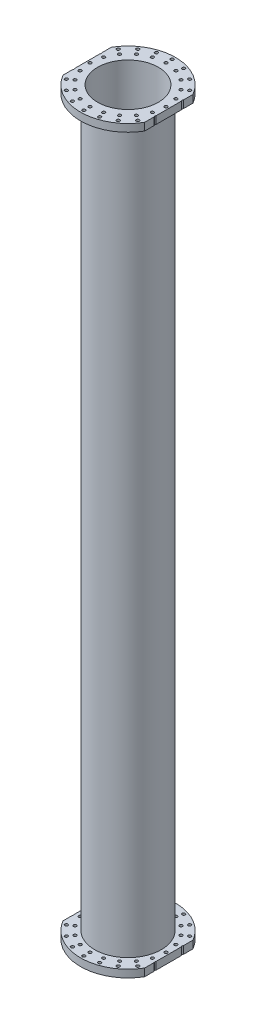
SolidWorks part; units mm, degrees
material "Q235B"
ref_plane "Front Plane" through (0, 0, 0) normal (0, 0, 1) x (1, 0, 0)
ref_plane "Top Plane" through (0, 0, 0) normal (0, 1, 0) x (1, 0, 0)
ref_plane "Right Plane" through (0, 0, 0) normal (1, 0, 0) x (0, 0, -1)
sketch "Sketch1" plane through (0, 0, 0) normal (0, 1, 0) x (1, 0, 0)
  line L1 (215, -400) -> (-215, -400)
  line L2 (215, -400) -> (215, 400)
  line L3 (215, 400) -> (-215, 400)
  line L4 (-215, -400) -> (-215, 400)
  line L5 (215, -400) -> (-215, 400) construction
  line L6 (215, 400) -> (-215, -400) construction
  circle A0 centre (0, 0) radius 250
  circle A1 centre (0, 0) radius 160
  dimension "D1" = 500
  dimension "D4" = 320
  dimension "D2" = 800
  dimension "D3" = 430
extrude "Boss-Extrude1" add sketch "Sketch1" along normal blind 40 contours L2 A0 L4 A1
sketch "Sketch2" plane through (0, 40, 0) normal (0, 1, 0) x (1, 0, 0)
  circle A0 centre (0, 0) radius 175.5
  circle A1 centre (0, 0) radius 160 construction
  circle A2 centre (0, 0) radius 160
  dimension "D1" = 351
extrude "Boss-Extrude2" add sketch "Sketch2" along normal blind 3817
hole_wizard "Ø16.0 (16) Diameter Hole1" positions "Sketch3" profile "Sketch4" hole size "Ø16.0" standard "GB" end condition up to next
sketch "Sketch3" plane through (0, 40, 0) normal (0, 1, 0) x (1, 0, 0)
  circle A0 centre (0, 0) radius 200 construction
  point P0 (200, 0)
  point P14 (190.2113, -61.8034)
  point P15 (161.8034, -117.5571)
  point P16 (117.5571, -161.8034)
  point P17 (61.8034, -190.2113)
  point P18 (0, -200)
  point P19 (-61.8034, -190.2113)
  point P20 (-117.5571, -161.8034)
  point P21 (-161.8034, -117.5571)
  point P22 (-190.2113, -61.8034)
  point P23 (-200, 0)
  point P24 (-190.2113, 61.8034)
  point P25 (-161.8034, 117.5571)
  point P26 (-117.5571, 161.8034)
  point P27 (-61.8034, 190.2113)
  point P28 (0, 200)
  point P29 (61.8034, 190.2113)
  point P30 (117.5571, 161.8034)
  point P31 (161.8034, 117.5571)
  point P32 (190.2113, 61.8034)
  point P36 (232.5, 0)
  point P45 (221.1206, -71.8465)
  point P46 (188.0965, -136.6601)
  point P47 (136.6601, -188.0965)
  point P48 (71.8465, -221.1206)
  point P49 (0, -232.5)
  point P50 (-71.8465, -221.1206)
  point P51 (-136.6601, -188.0965)
  point P52 (-188.0965, -136.6601)
  point P53 (-221.1206, -71.8465)
  point P54 (-232.5, 0)
  point P55 (-221.1206, 71.8465)
  point P56 (-188.0965, 136.6601)
  point P57 (-136.6601, 188.0965)
  point P58 (-71.8465, 221.1206)
  point P59 (0, 232.5)
  point P60 (71.8465, 221.1206)
  point P61 (136.6601, 188.0965)
  point P62 (188.0965, 136.6601)
  point P63 (221.1206, 71.8465)
  dimension "D1" = 400
  dimension "D3" = 232.5
  dimension "D2" = 20
  dimension "D4" = 20
sketch "Sketch4" plane through (200, 40, 0) normal (1, 0, 0) x (0, 0, 1)
  line L0 (0, 0) -> (0, 40)
  line L1 (0, 40) -> (8, 40)
  line L2 (8, 40) -> (8, 0)
  line L5 (8, 0) -> (0, 0)
  line L11 (0, -6.35) -> (0, 107.95) construction
  dimension "通孔孔直径" = 16
  dimension "通孔孔深度" = 40
pattern_linear "LPattern1" count 2 spacing 3857 along (0, 1, 0) of "Ø16.0 (16) Diameter Hole1", "Boss-Extrude1"
